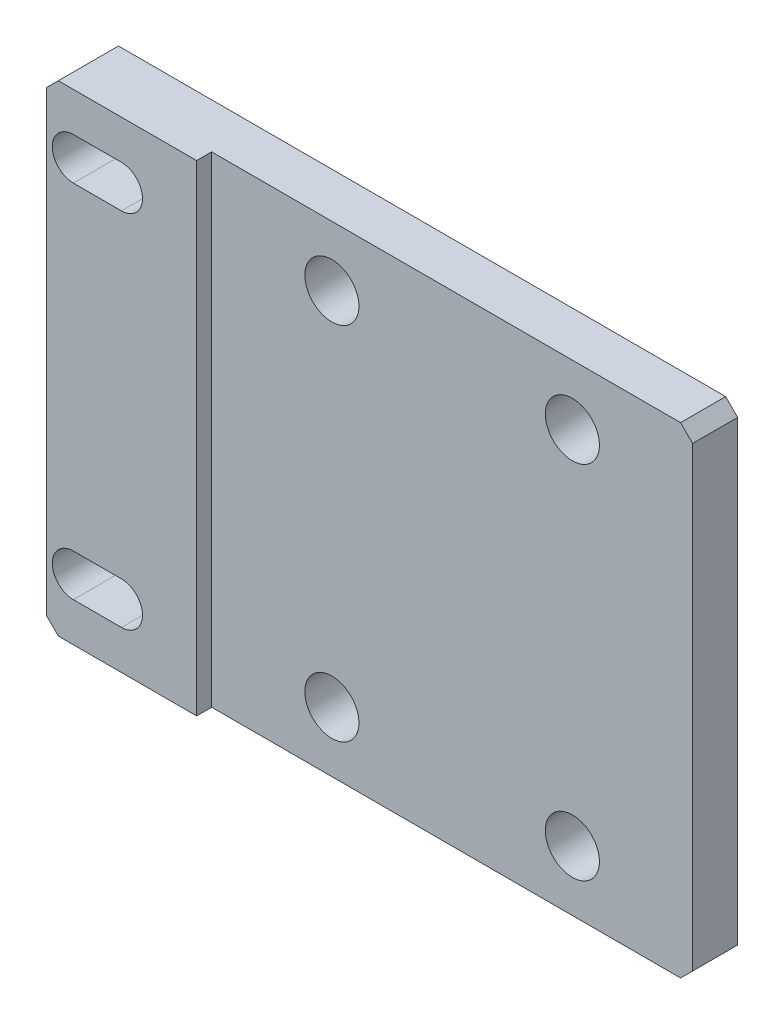
from build123d import *

# Parameters (mm, degrees)
SKETCH_1_W             = 105
SKETCH_1_H             = 80
EXTRUDE_1_DEPTH        = 5
SKETCH_2_W             = 80
SKETCH_2_H             = 80
CUT_EXTRUDE_1_DEPTH    = 2.5
HOLE_WIZARD_9_0_9_1_D  = 9
HOLE_WIZARD_7_0_7_1_D  = 7
CHAMFER_1_SIZE         = 2
CUT_EXTRUDE_3_DEPTH    = 10
PATTERN_LINEAR_1_COUNT = 2
PATTERN_LINEAR_1_PITCH = 60


with BuildPart() as part:
    # 草图1 → 凸台-拉伸1 (new, symmetric)
    with BuildSketch(Plane.XY):
        Rectangle(SKETCH_1_W, SKETCH_1_H)
    extrude(amount=EXTRUDE_1_DEPTH, both=True)

    # 草图2 → 切除-拉伸1 (cut)
    with BuildSketch(Plane.XY.offset(5)):
        with Locations((12.5, 0)):
            Rectangle(SKETCH_2_W, SKETCH_2_H)
    extrude(amount=-CUT_EXTRUDE_1_DEPTH, mode=Mode.SUBTRACT)

    # Ø9.0 (9) 直径孔1 (through all)
    with Locations(Plane.XY.offset(5)):
        with Locations((-7.5, 30), (32.5, 30), (32.5, -30), (-7.5, -30)):
            Hole(HOLE_WIZARD_9_0_9_1_D / 2)

    # Ø7.0 (7) 直径孔1 (through all)
    with Locations(Plane.XY.offset(5)):
        with Locations((-44, 30), (-86, 30), (-44, -30), (-86, -30)):
            Hole(HOLE_WIZARD_7_0_7_1_D / 2)

    # 倒角1
    chamfer_1_edges = [part.edges().sort_by_distance(p)[0] for p in [
        (52.5, -40, -1.25),
        (52.5, 40, -1.25),
        (-52.5, -40, 0),
        (-52.5, 40, 0),
    ]]
    chamfer(chamfer_1_edges, length=CHAMFER_1_SIZE)

    # 草图8 → 切除-拉伸3 (cut)
    with BuildSketch(Plane.XY.offset(5)):
        with BuildLine():
            Line((-40, 26.5), (-48, 26.5))
            ThreePointArc((-48, 26.5), (-51.5, 30), (-48, 33.5))
            Line((-48, 33.5), (-40, 33.5))
            ThreePointArc((-40, 33.5), (-36.5, 30), (-40, 26.5))
        make_face()
    cut_extrude_3 = extrude(amount=-CUT_EXTRUDE_3_DEPTH, mode=Mode.SUBTRACT)

    # 阵列(线性)1: 切除-拉伸3 ×2
    with Locations(*[(0, -i * PATTERN_LINEAR_1_PITCH, 0) for i in range(1, PATTERN_LINEAR_1_COUNT)]):
        add(cut_extrude_3, mode=Mode.SUBTRACT)


solid = part.part
